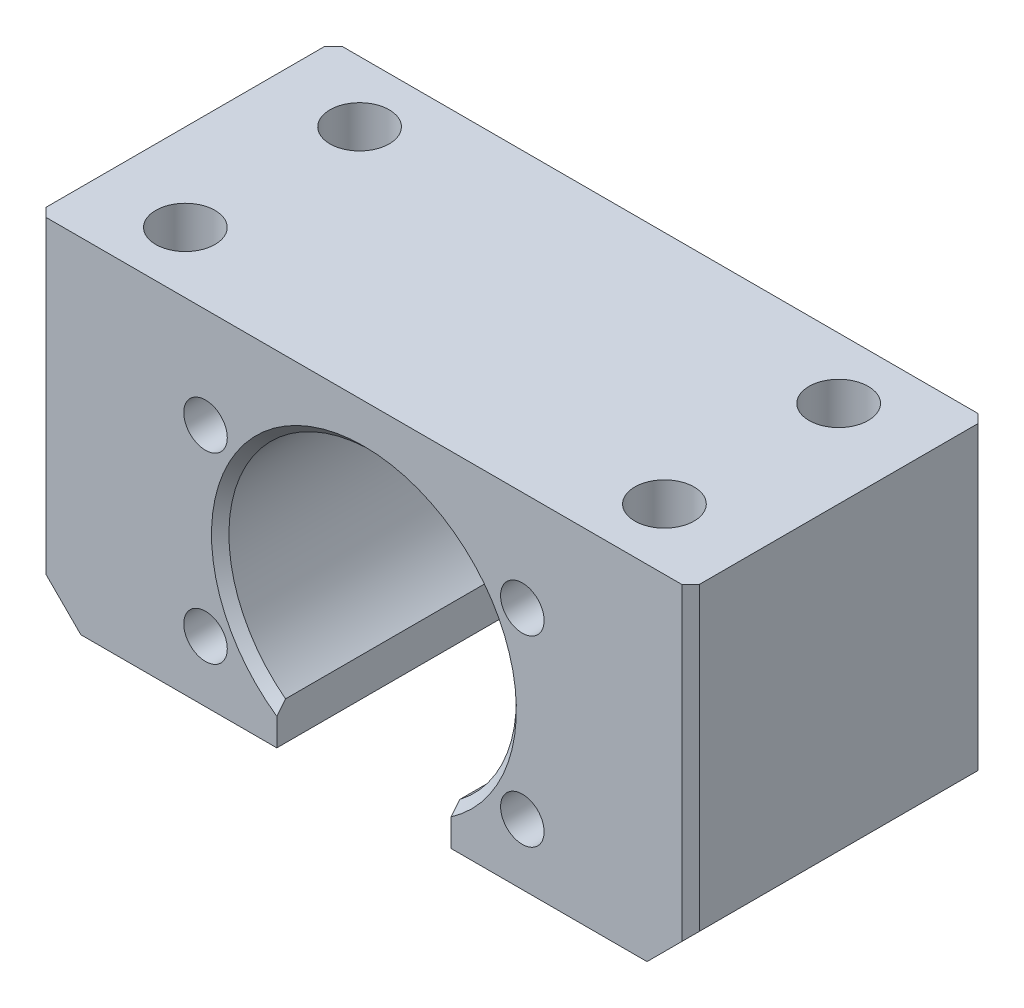
SolidWorks part; units mm, degrees
material "Q235A"
ref_plane "前视基准面" through (0, 0, 0) normal (0, 0, 1) x (1, 0, 0)
ref_plane "上视基准面" through (0, 0, 0) normal (0, 1, 0) x (1, 0, 0)
ref_plane "右视基准面" through (0, 0, 0) normal (1, 0, 0) x (0, 0, -1)
sketch "草图1" plane through (0, 0, 0) normal (0, 0, 1) x (1, 0, 0)
  line L1 (-37.5, -19.75) -> (37.5, -19.75)
  line L2 (-37.5, -19.75) -> (-37.5, 19.75)
  line L3 (-37.5, 19.75) -> (37.5, 19.75)
  line L4 (37.5, -19.75) -> (37.5, 19.75)
  line L5 (-37.5, -19.75) -> (37.5, 19.75) construction
  line L6 (-37.5, 19.75) -> (37.5, -19.75) construction
  point P0 (0, 0)
  dimension "D1" = 75
  dimension "D2" = 39.5
extrude "凸台-拉伸1" add sketch "草图1" along normal blind 34
sketch "草图2" plane through (0, 0, 34) normal (0, 0, 1) x (1, 0, 0)
  line L0 (-37.5, -19.75) -> (37.5, -19.75) construction
  circle A0 centre (0, -2.25) radius 16.5
  dimension "D1" = 33
  dimension "D2" = 1
extrude "切除-拉伸1" cut sketch "草图2" against normal through all
sketch "草图3" plane through (0, 0, 34) normal (0, 0, 1) x (1, 0, 0)
  line L0 (-37.5, -19.75) -> (37.5, -19.75) construction
  line L1 (-10, -15.3744) -> (10, -15.3744)
  line L2 (-10, -15.3744) -> (-10, -19.75)
  line L3 (-10, -19.75) -> (10, -19.75)
  line L4 (10, -15.3744) -> (10, -19.75)
  circle A0 centre (0, -2.25) radius 16.5 construction
  dimension "D1" = 20
extrude "切除-拉伸2" cut sketch "草图3" against normal through all
hole_wizard "M5 螺纹孔1" positions "草图4" profile "草图5" tap size "M5" standard "ISO"
sketch "草图4" plane through (0, 0, 30) normal (0, 0, 1) x (1, 0, 0)
  line L0 (0, 0) -> (0, 28.46) construction
  line L3 (0, -14.75) -> (28.8824, -14.75) construction
  point P0 (-20, -14.75)
  point P2 (20, -14.75)
  dimension "D1" = 40
sketch "草图5" plane through (-20, -14.75, 30) normal (1, 0, 0) x (0, -1, 0)
  line L0 (0, 0) -> (0, 30)
  line L1 (0, 30) -> (2.1, 30)
  line L2 (2.1, 30) -> (2.1, 0)
  line L5 (2.1, 0) -> (0, 0)
  line L11 (0, -6.35) -> (0, 107.95) construction
  dimension "通孔螺纹孔钻头直径" = 4.2
  dimension "通孔螺纹孔钻头深度" = 30
cosmetic thread "孔螺蚊线1" [suppressed] parameters "D2"=5
cosmetic thread "孔螺蚊线2" [suppressed] parameters "D2"=5
hole_wizard "M8 螺纹孔1" positions "草图6" profile "草图7" tap size "M8" standard "ISO"
sketch "草图6" plane through (0, 19.75, 0) normal (0, 1, 0) x (1, 0, 0)
  line L0 (0, 0) -> (0, -34) construction
  line L1 (37.5, -34) -> (-37.5, -34) construction
  line L3 (-37.5, -17) -> (37.5, -17) construction
  line L4 (-37.5, -34) -> (-37.5, 0) construction
  line L5 (37.5, -34) -> (37.5, 0) construction
  point P0 (-27.5, -7)
  point P2 (-27.5, -27)
  point P20 (27.5, -27)
  point P21 (27.5, -7)
  dimension "D1" = 20
  dimension "D2" = 55
sketch "草图7" plane through (-27.5, 19.75, 7) normal (1, 0, 0) x (0, 0, 1)
  line L0 (0, 0) -> (0, 21.7929)
  line L1 (0, 21.7929) -> (3.4, 19.75)
  line L2 (3.4, 19.75) -> (3.4, 0)
  line L5 (3.4, 0) -> (0, 0)
  line L10 (0, 21.7929) -> (-3.4, 19.75) construction
  line L11 (0, -6.35) -> (0, 107.95) construction
  dimension "螺纹孔钻头直径" = 6.8
  dimension "螺纹孔钻头深度" = 19.75
  dimension "导头角度" = 118
cosmetic thread "孔螺蚊线3" parameters "D1"=16, "D2"=8
cosmetic thread "孔螺蚊线4" parameters "D1"=16, "D2"=8
cosmetic thread "孔螺蚊线5" parameters "D1"=16, "D2"=8
cosmetic thread "孔螺蚊线6" parameters "D1"=16, "D2"=8
chamfer "倒角1" distance 5 angle 45 2 edges at (37.5, -19.75, 17) (-37.5, -19.75, 17)
chamfer "倒角2" distance 1 angle 45 6 edges at (0, 14.25, 0) (0, 14.25, 34) (37.5, 2.5, 34) (37.5, 2.5, 0) (-37.5, 2.5, 0) (-37.5, 2.5, 34)
hole_wizard "M6 螺纹孔1" positions "草图8" profile "草图9" tap size "M6" standard "ISO"
sketch "草图8" plane through (0, 0, 34) normal (0, 0, 1) x (1, 0, 0)
  arc A0 (10, -15.3744) -> (-10, -15.3744) centre (0, -2.25) ccw construction
  point P0 (-18.1865, 8.25)
  point P3 (-18.1865, -12.75)
  point P6 (18.1865, 8.25)
  point P9 (18.1865, -12.75)
  dimension "D1" = 18.1865
  dimension "D2" = 18.1865
  dimension "D3" = 10.5
  dimension "D4" = 10.5
cosmetic thread "孔螺蚊线8" parameters "D1"=12, "D2"=6
cosmetic thread "孔螺蚊线10" parameters "D1"=12, "D2"=6
cosmetic thread "孔螺蚊线11" parameters "D1"=12, "D2"=6
cosmetic thread "孔螺蚊线12" parameters "D1"=12, "D2"=6
sketch "草图9" plane through (-18.1865, 8.25, 34) normal (1, 0, 0) x (0, -1, 0)
  line L0 (0, 0) -> (0, 16.5022)
  line L1 (0, 16.5022) -> (2.5, 15)
  line L2 (2.5, 15) -> (2.5, 0)
  line L5 (2.5, 0) -> (0, 0)
  line L10 (0, 16.5022) -> (-2.5, 15) construction
  line L11 (0, -6.35) -> (0, 107.95) construction
  dimension "螺纹孔钻头直径" = 5
  dimension "螺纹孔钻头深度" = 15
  dimension "导头角度" = 118
